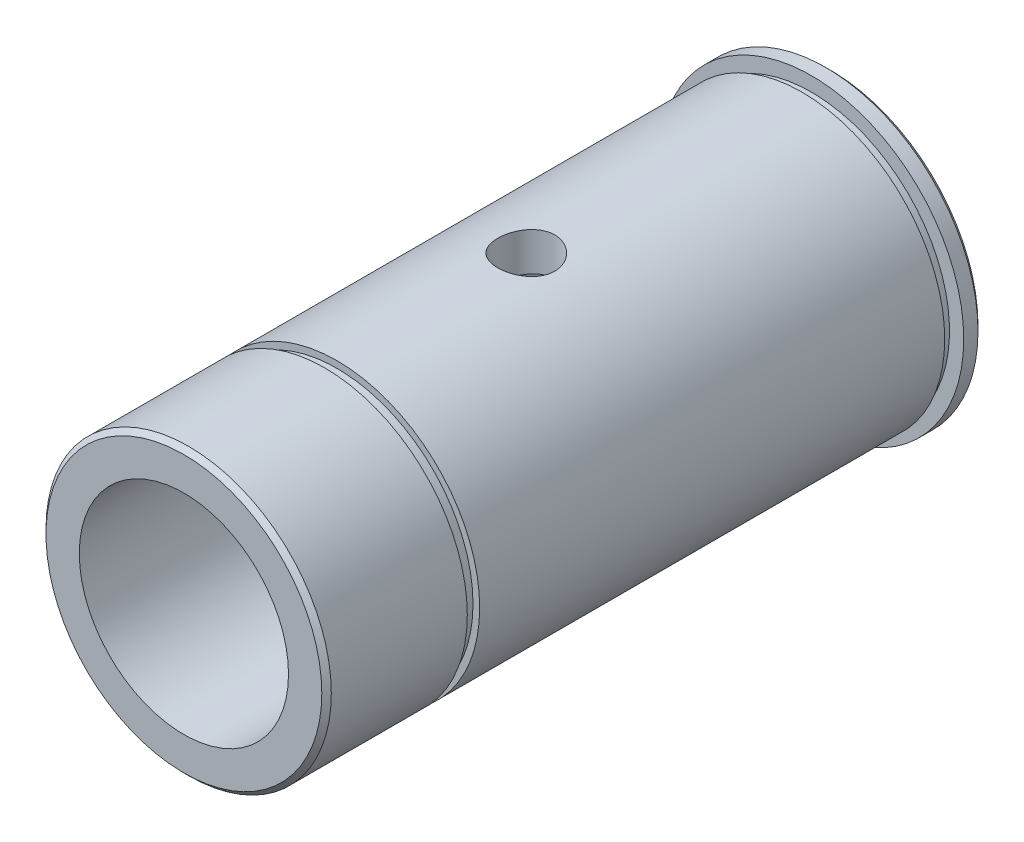
from build123d import *

# Parameters (mm, degrees)
SKETCH_1_R          = 16
EXTRUDE_1_DEPTH     = 2
SKETCH_2_R          = 15
EXTRUDE_2_DEPTH     = 66
SKETCH_3_R          = 9
CUT_EXTRUDE_1_DEPTH = 72.665891469
SKETCH_5_R          = 11
CUT_EXTRUDE_2_DEPTH = 66
SKETCH_8_R          = 3
CUT_EXTRUDE_3_DEPTH = 10
SKETCH_9_W          = 1.3
SKETCH_9_H          = 0.7
CHAMFER_1_SIZE      = 0.5
SKETCH_10_W         = 0.5
SKETCH_10_H         = 1


with BuildPart() as part:
    # 草图1 → 凸台-拉伸1 (new body)
    with BuildSketch(Plane.XY):
        Circle(SKETCH_1_R)
    extrude(amount=EXTRUDE_1_DEPTH)

    # 草图2 → 凸台-拉伸2 (add)
    with BuildSketch(Plane.XY.offset(2)):
        Circle(SKETCH_2_R)
    extrude(amount=EXTRUDE_2_DEPTH)

    # 草图3 → 切除-拉伸1 (cut, through all)
    with BuildSketch(Plane(origin=(0, 0, 0), x_dir=(-1, 0, 0), z_dir=(0, 0, -1))):
        Circle(SKETCH_3_R)
    extrude(amount=-CUT_EXTRUDE_1_DEPTH, mode=Mode.SUBTRACT)

    # 草图5 → 切除-拉伸2 (cut)
    with BuildSketch(Plane.XY.offset(68)):
        Circle(SKETCH_5_R)
    extrude(amount=-CUT_EXTRUDE_2_DEPTH, mode=Mode.SUBTRACT)

    # 草图8 → 切除-拉伸3 (cut)
    with BuildSketch(Plane(origin=(0, 15, 0), x_dir=(1, 0, 0), z_dir=(0, 1, 0))):
        with Locations(Location((0, -32, 0), (0, 0, 270))):
            Circle(SKETCH_8_R)
    extrude(amount=-CUT_EXTRUDE_3_DEPTH, mode=Mode.SUBTRACT)

    # 草图9 → 切除-旋转1 (revolve, cut)
    with BuildSketch(Plane(origin=(0, 0, 0), x_dir=(0, 0, -1), z_dir=(1, 0, 0)), mode=Mode.PRIVATE) as cut_revolve_1_sk:
        with Locations((-52.55, 14.65)):
            Rectangle(SKETCH_9_W, SKETCH_9_H)
    revolve(cut_revolve_1_sk.sketch.rotate(Axis((0, 0, 68), (0, 0, -1)), 90), axis=Axis((0, 0, 68), (0, 0, -1)), mode=Mode.SUBTRACT)

    # 倒角1
    chamfer_1_edges = [part.edges().sort_by_distance(p)[0] for p in [
        (-16, 0, 0),
        (-15, 0, 68),
    ]]
    chamfer(chamfer_1_edges, length=CHAMFER_1_SIZE)

    # 草图10 → 切除-旋转2 (revolve, cut)
    with BuildSketch(Plane(origin=(0, 0, 0), x_dir=(1, 0, 0), z_dir=(0, 1, 0))):
        with Locations((-14.75, -2.5)):
            Rectangle(SKETCH_10_W, SKETCH_10_H)
    revolve(axis=Axis((0, 0, 0), (0, 0, 1)), mode=Mode.SUBTRACT)


solid = part.part
